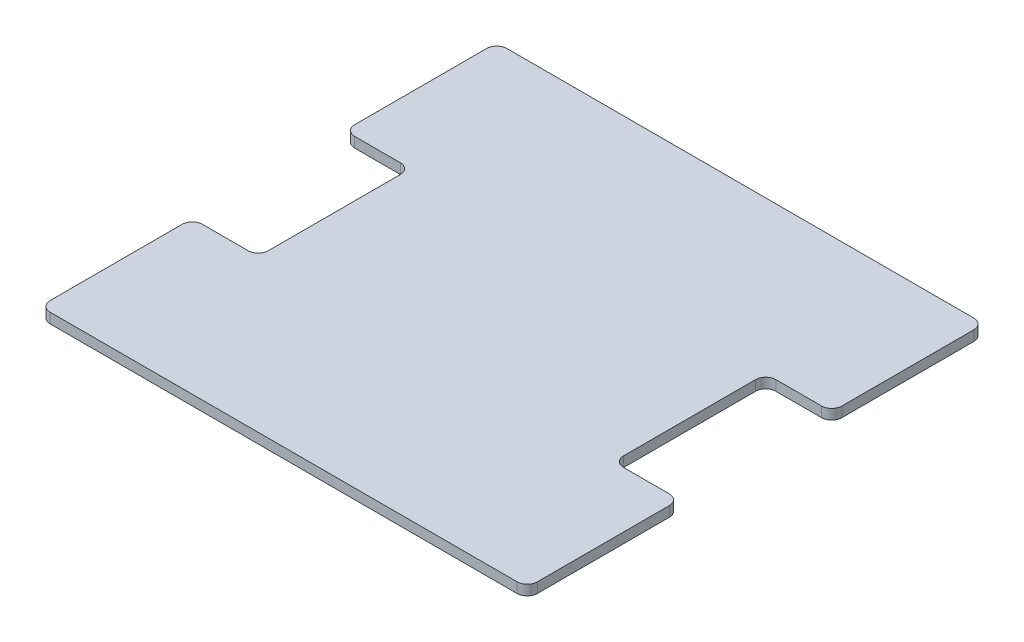
SolidWorks part; units mm, degrees
ref_plane "Front Plane" through (0, 0, 0) normal (0, 0, 1) x (1, 0, 0)
ref_plane "Top Plane" through (0, 0, 0) normal (0, 1, 0) x (1, 0, 0)
ref_plane "Right Plane" through (0, 0, 0) normal (1, 0, 0) x (0, 0, -1)
other "Configuration Table"
sketch "Sketch1" plane through (0, 0, 0) normal (0, 1, 0) x (1, 0, 0)
  line L1 (-240, 325) -> (240, 325)
  line L2 (-240, 325) -> (-240, -325)
  line L3 (-240, -325) -> (240, -325)
  line L4 (240, 325) -> (240, -325)
  line L5 (-240, 325) -> (240, -325) construction
  line L6 (-240, -325) -> (240, 325) construction
  point P0 (0, 0)
  dimension "D1" = 650
  dimension "D2" = 480
extrude "Boss-Extrude1" add sketch "Sketch1" along normal blind 10
sketch "Sketch3" plane through (0, 10, 0) normal (0, 1, 0) x (1, 0, 0)
  line L0 (0, 325) -> (0, -325) construction
  line L1 (240, 325) -> (-240, 325) construction
  line L2 (-240, -325) -> (240, -325) construction
  line L3 (-240, 0) -> (240, 0) construction
  line L4 (-240, 325) -> (-240, -325) construction
  line L5 (240, -325) -> (240, 325) construction
  line L6 (0, -325) -> (0, -225)
  line L8 (220, -255) -> (175, -255)
  line L9 (-220, -195) -> (-175, -195)
  line L10 (-220, -195) -> (-220, -255)
  line L11 (-220, -255) -> (-175, -255)
  line L12 (-175, -195) -> (-175, -255)
  line L13 (-220, -195) -> (-175, -255) construction
  line L14 (-220, -255) -> (-175, -195) construction
  line L15 (220, -195) -> (175, -195)
  line L16 (220, -195) -> (220, -255)
  line L17 (175, -195) -> (175, -255)
  line L18 (220, 255) -> (175, 255)
  line L19 (220, 195) -> (175, 195)
  line L20 (220, 195) -> (220, 255)
  line L21 (175, 195) -> (175, 255)
  line L22 (-220, 255) -> (-175, 255)
  line L23 (-175, 195) -> (-175, 255)
  line L24 (-220, 195) -> (-220, 255)
  line L25 (-220, 195) -> (-175, 195)
  line L26 (305, -75) -> (175, -75)
  line L27 (-305, 75) -> (-175, 75)
  line L28 (-305, 75) -> (-305, -75)
  line L29 (-305, -75) -> (-175, -75)
  line L30 (-175, 75) -> (-175, -75)
  line L31 (-305, 75) -> (-175, -75) construction
  line L32 (-305, -75) -> (-175, 75) construction
  line L33 (175, 75) -> (175, -75)
  line L34 (305, 75) -> (175, 75)
  line L35 (305, 75) -> (305, -75)
  dimension "D2" = 60
  dimension "D3" = 45
  dimension "D4" = 150
  dimension "D5" = 130
fillet "Fillet2" radius 60 4 edges at (-240, 5, -325) (240, 5, -325) (240, 5, 325) (-240, 5, 325)
extrude "Cut-Extrude1" cut sketch "Sketch3" against normal blind 10 contours L28 L29 L30 L27 | L35 L26 L33 L34
sketch "Sketch5" plane through (0, 10, 0) normal (0, 1, 0) x (1, 0, 0)
  line L0 (281.3781, -325) -> (281.3781, -225)
  line L1 (299.7696, 0) -> (-274.5789, 0) construction
  line L2 (-281.3781, -225) -> (281.3781, -225)
  line L3 (-281.3781, 325) -> (281.3781, 325)
  line L4 (-281.3781, 325) -> (-281.3781, 225)
  line L5 (-281.3781, 225) -> (281.3781, 225)
  line L6 (281.3781, 325) -> (281.3781, 225)
  line L7 (-281.3781, 325) -> (281.3781, 225) construction
  line L8 (-281.3781, 225) -> (281.3781, 325) construction
  line L9 (-281.3781, -325) -> (281.3781, -325)
  line L10 (-281.3781, -325) -> (-281.3781, -225)
  dimension "D2" = 100
extrude "Cut-Extrude2" cut sketch "Sketch5" against normal blind 10
fillet "Fillet3" radius 10 12 edges at (-240, 5, -225) (240, 5, -225) (240, 5, -75) (175, 5, -75) (175, 5, 75) (240, 5, 75) (240, 5, 225) (-240, 5, 225) (-240, 5, 75) (-175, 5, 75) (-175, 5, -75) (-240, 5, -75)
